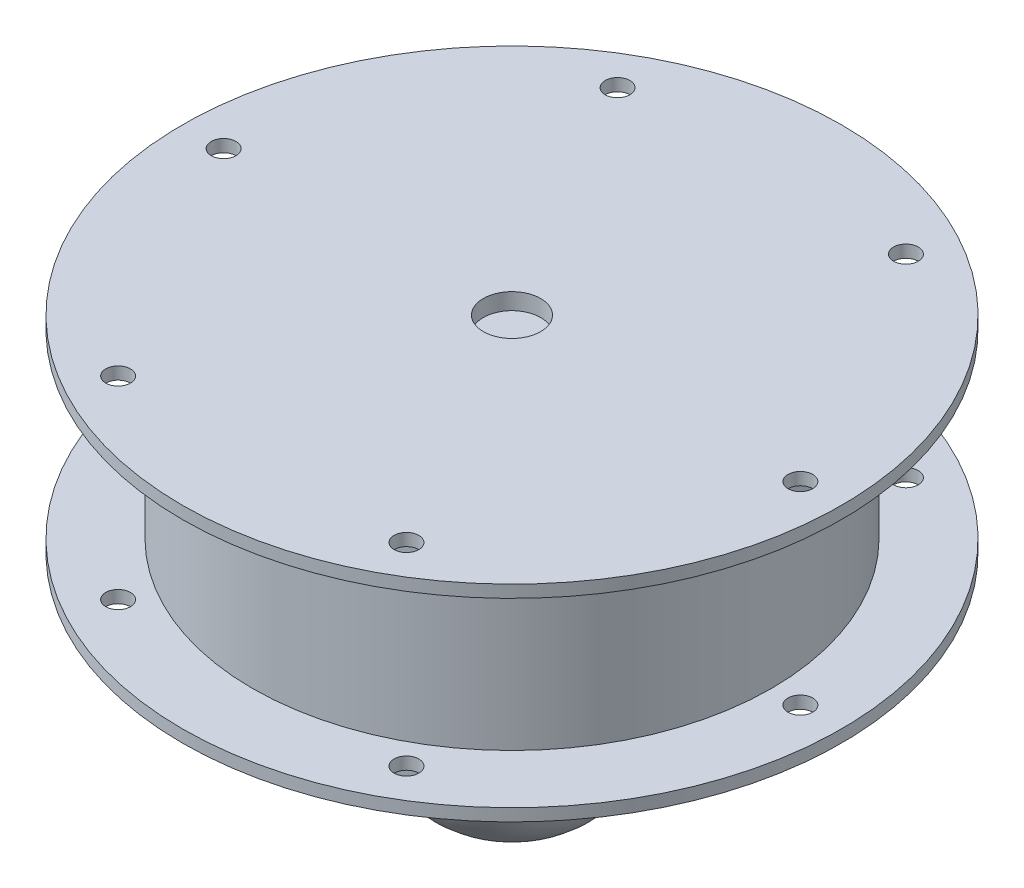
from build123d import *

# Parameters (mm, degrees)
SKETCH2_R           = 1.5
CUT_EXTRUDE1_DEPTH  = 62.846584384
SKETCH3_R           = 30
BOSS_EXTRUDE1_DEPTH = 2
SKETCH4_R           = 3.481990468
CUT_EXTRUDE2_DEPTH  = 2
SKETCH5_R           = 17.5
BOSS_EXTRUDE2_DEPTH = 35
SKETCH6_R           = 13
BOSS_EXTRUDE3_DEPTH = 15
FILLET1_R           = 12


with BuildPart() as part:
    # Sketch1 → Revolve1 (revolve)
    with BuildSketch(Plane.XY, mode=Mode.PRIVATE) as revolve1_sk:
        Polygon((-40, 0), (-30, 0), (-30, 25), (-40, 25), (-40, 23.5), (-31.5, 23.5), (-31.5, 1.5), (-40, 1.5), align=None)
    revolve(revolve1_sk.sketch.rotate(Axis((0, 0, 0), (0, 1, 0)), 270), axis=Axis((0, 0, 0), (0, 1, 0)))

    # Sketch2 → Cut-Extrude1 (cut, through all)
    with BuildSketch(Plane(origin=(0, 25, 0), x_dir=(1, 0, 0), z_dir=(0, 1, 0))):
        with Locations(Location((-35, 0, 0), (0, 0, 270))):
            Circle(SKETCH2_R)
        with Locations(Location((-17.5, 30.310889132, 0), (0, 0, 270))):
            Circle(SKETCH2_R)
        with Locations(Location((17.5, 30.310889132, 0), (0, 0, 270))):
            Circle(SKETCH2_R)
        with Locations(Location((35, 0, 0), (0, 0, 270))):
            Circle(SKETCH2_R)
        with Locations(Location((17.5, -30.310889132, 0), (0, 0, 270))):
            Circle(SKETCH2_R)
        with Locations(Location((-17.5, -30.310889132, 0), (0, 0, 270))):
            Circle(SKETCH2_R)
    extrude(amount=-CUT_EXTRUDE1_DEPTH, mode=Mode.SUBTRACT)

    # Sketch3 → Boss-Extrude1 (add)
    with BuildSketch(Plane(origin=(0, 25, 0), x_dir=(1, 0, 0), z_dir=(0, 1, 0))):
        with Locations(Location((0, 0, 0), (0, 0, 90))):
            Circle(SKETCH3_R)
    extrude(amount=-BOSS_EXTRUDE1_DEPTH)

    # Sketch4 → Cut-Extrude2 (cut)
    with BuildSketch(Plane(origin=(0, 23, 0), x_dir=(-1, 0, 0), z_dir=(0, -1, 0))):
        with Locations(Location((0, 0, 0), (0, 0, 90))):
            Circle(SKETCH4_R)
    extrude(amount=-CUT_EXTRUDE2_DEPTH, mode=Mode.SUBTRACT)

    # Sketch5 → Boss-Extrude2 (add)
    with BuildSketch(Plane(origin=(0, 23, 0), x_dir=(-1, 0, 0), z_dir=(0, -1, 0))):
        with Locations(Location((0, 0, 0), (0, 0, 270))):
            Circle(SKETCH5_R)
    extrude(amount=BOSS_EXTRUDE2_DEPTH)

    # Sketch6 → Boss-Extrude3 (add)
    with BuildSketch(Plane(origin=(0, -12, 0), x_dir=(-1, 0, 0), z_dir=(0, -1, 0))):
        with Locations(Location((0, 0, 0), (0, 0, 90))):
            Circle(SKETCH6_R)
    extrude(amount=BOSS_EXTRUDE3_DEPTH)

    # Fillet1
    fillet1_edges = [part.edges().sort_by_distance(p)[0] for p in [
        (0, -27, 13),
    ]]
    fillet(fillet1_edges, radius=FILLET1_R)


solid = part.part
